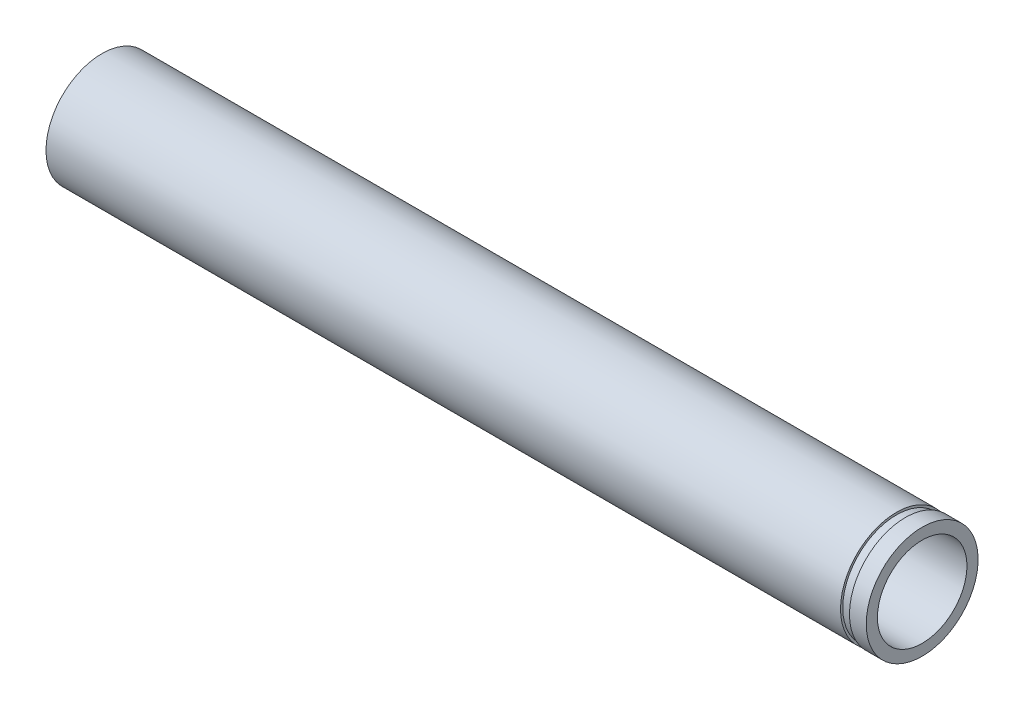
from build123d import *

# Parameters (mm, degrees)
EXTRUDE_START   = 200
SKETCH_3_R      = 50
SKETCH_3_R_2    = 40
EXTRUDE_1_DEPTH = 200
EXTRUDE_START_2 = -8
SKETCH_4_R      = 40
SKETCH_4_R_2    = 25
EXTRUDE_2_DEPTH = 8


with BuildPart() as part:
    # 草图2 → 旋转1 (revolve)
    with BuildSketch(Plane.XY, mode=Mode.PRIVATE) as revolve_1_sk:
        Polygon((-22.357142857, 40), (532.642857143, 40), (532.642857143, 50), (517.642857143, 50), (517.642857143, 48), (509.642857143, 48), (509.642857143, 50), (-0.617142857, 50), (-0.617142857, 48), (-8.617142857, 48), (-8.617142857, 50), (-22.357142857, 50), align=None)
    revolve(revolve_1_sk.sketch.rotate(Axis((-27.214285714, 0, 0), (1, 0, 0)), 90), axis=Axis((-27.214285714, 0, 0), (1, 0, 0)))

    # 草图3 → 凸台-拉伸1 (add)
    with BuildSketch(Plane.ZY.offset(0.617142857).offset(EXTRUDE_START)):
        Circle(SKETCH_3_R)
        Circle(SKETCH_3_R_2, mode=Mode.SUBTRACT)
    extrude(amount=-EXTRUDE_1_DEPTH)

    # 草图4 → 凸台-拉伸2 (add)
    with BuildSketch(Plane.ZY.offset(200.617142857).offset(EXTRUDE_START_2)):
        Circle(SKETCH_4_R)
        Circle(SKETCH_4_R_2, mode=Mode.SUBTRACT)
    extrude(amount=EXTRUDE_2_DEPTH)


solid = part.part
